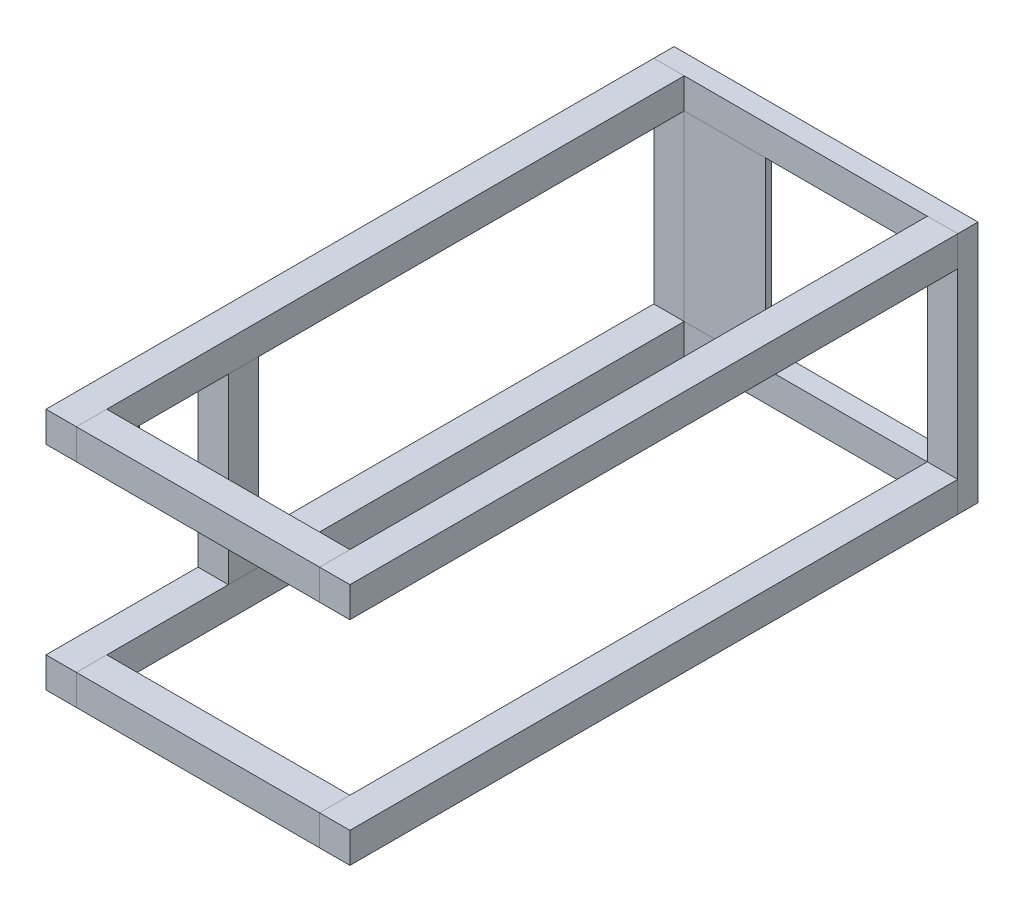
from build123d import *

# Parameters (mm, degrees)
SKETCH2_W               = 150
SKETCH2_H               = 120
BOSS_EXTRUDE1_DEPTH     = 10
CUT_EXTRUDE4_DEPTH      = 97.566039579
CUT_EXTRUDE4_DEPTH_BACK = 97.566039579
SKETCH6_W               = 120
SKETCH6_H               = 90
SKETCH7_W               = 15
SKETCH7_H               = 15
BOSS_EXTRUDE2_DEPTH     = 300
BOSS_EXTRUDE2_2_DEPTH   = 300
BOSS_EXTRUDE2_3_DEPTH   = 300
BOSS_EXTRUDE2_4_DEPTH   = 300
SKETCH14_W              = 15
SKETCH14_H              = 15
BOSS_EXTRUDE7_DEPTH     = 120
BOSS_EXTRUDE7_2_DEPTH   = 120
SKETCH15_W              = 15
SKETCH15_H              = 15
BOSS_EXTRUDE8_DEPTH     = 90
SKETCH16_R              = 2.5
BOSS_EXTRUDE9_DEPTH     = 14
SKETCH17_W              = 40
SKETCH17_H              = 90
BOSS_EXTRUDE10_DEPTH    = 3


with BuildPart() as part:
    # Sketch2 → Boss-Extrude1 (new body)
    with BuildSketch(Plane.XY):
        Rectangle(SKETCH2_W, SKETCH2_H)
    extrude(amount=BOSS_EXTRUDE1_DEPTH)

    # Sketch6 → Cut-Extrude4 (cut, two sides: drawn at the far end of the back side and taken through both)
    with BuildSketch(Plane.XY.offset(10).offset(-CUT_EXTRUDE4_DEPTH_BACK)):
        Rectangle(SKETCH6_W, SKETCH6_H)
    extrude(amount=CUT_EXTRUDE4_DEPTH + CUT_EXTRUDE4_DEPTH_BACK, mode=Mode.SUBTRACT)


with BuildPart() as body_2:
    # Sketch7 → Boss-Extrude2 (new body)
    with BuildSketch(Plane.XY.offset(10)):
        with Locations((-67.5, 52.5)):
            Rectangle(SKETCH7_W, SKETCH7_H)
    extrude(amount=BOSS_EXTRUDE2_DEPTH)

    # Sketch16 → Boss-Extrude9 (add)
    with BuildSketch(Plane.XZ.offset(-45)):
        with Locations(Location((-67.5, 275, 0), (0, 0, 180))):
            Circle(SKETCH16_R)
    extrude(amount=BOSS_EXTRUDE9_DEPTH)


with BuildPart() as body_3:
    # Sketch7 → Boss-Extrude2 2 (new body)
    with BuildSketch(Plane.XY.offset(10)):
        with Locations((-67.5, -52.5)):
            Rectangle(SKETCH7_W, SKETCH7_H)
    extrude(amount=BOSS_EXTRUDE2_2_DEPTH)


with BuildPart() as body_4:
    # Sketch7 → Boss-Extrude2 3 (new body)
    with BuildSketch(Plane.XY.offset(10)):
        with Locations((67.5, 52.5)):
            Rectangle(SKETCH7_W, SKETCH7_H)
    extrude(amount=BOSS_EXTRUDE2_3_DEPTH)


with BuildPart() as body_5:
    # Sketch7 → Boss-Extrude2 4 (new body)
    with BuildSketch(Plane.XY.offset(10)):
        with Locations((67.5, -52.5)):
            Rectangle(SKETCH7_W, SKETCH7_H)
    extrude(amount=BOSS_EXTRUDE2_4_DEPTH)


with BuildPart() as body_6:
    # Sketch14 → Boss-Extrude7 (new body)
    with BuildSketch(Plane(origin=(-60, 0, 0), x_dir=(0, 0, -1), z_dir=(1, 0, 0))):
        with Locations((-302.5, 52.5)):
            Rectangle(SKETCH14_W, SKETCH14_H)
    extrude(amount=BOSS_EXTRUDE7_DEPTH)


with BuildPart() as body_7:
    # Sketch14 → Boss-Extrude7 2 (new body)
    with BuildSketch(Plane(origin=(-60, 0, 0), x_dir=(0, 0, -1), z_dir=(1, 0, 0))):
        with Locations((-302.5, -52.5)):
            Rectangle(SKETCH14_W, SKETCH14_H)
    extrude(amount=BOSS_EXTRUDE7_2_DEPTH)


with BuildPart() as body_8:
    # Sketch15 → Boss-Extrude8 (new body)
    with BuildSketch(Plane.XZ.offset(-45)):
        with Locations((-67.5, 227.5)):
            Rectangle(SKETCH15_W, SKETCH15_H)
    extrude(amount=BOSS_EXTRUDE8_DEPTH)


with BuildPart() as body_9:
    # Sketch17 → Boss-Extrude10 (new body)
    with BuildSketch(Plane.XY.offset(10)):
        with Locations((-40, 0)):
            Rectangle(SKETCH17_W, SKETCH17_H)
    extrude(amount=-BOSS_EXTRUDE10_DEPTH)


solid = Compound([part.part, body_2.part, body_3.part, body_4.part, body_5.part, body_6.part, body_7.part, body_8.part, body_9.part])
